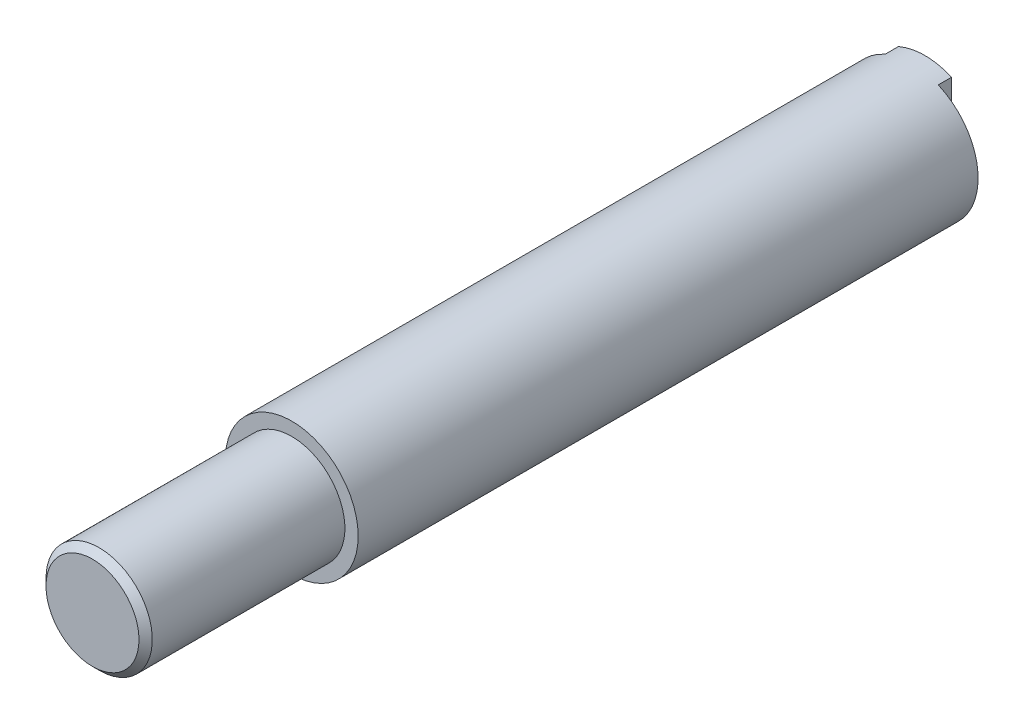
SolidWorks part; units mm, degrees
ref_plane "Front Plane" through (0, 0, 0) normal (0, 0, 1) x (1, 0, 0)
ref_plane "Top Plane" through (0, 0, 0) normal (0, 1, 0) x (1, 0, 0)
ref_plane "Right Plane" through (0, 0, 0) normal (1, 0, 0) x (0, 0, -1)
sketch "Sketch1" plane through (0, 0, 0) normal (0, 0, 1) x (1, 0, 0)
  circle A0 centre (0, 0) radius 15
  dimension "D1" = 30
extrude "Boss-Extrude1" add sketch "Sketch1" along normal blind 140
sketch "Sketch2" plane through (0, 0, 140) normal (0, 0, 1) x (1, 0, 0)
  circle A0 centre (0, 0) radius 12
  dimension "D1" = 24
extrude "Boss-Extrude2" add sketch "Sketch2" along normal blind 45
sketch "Sketch3" plane through (0, 0, 0) normal (0, 0, -1) x (-1, 0, 0)
  line L0 (0, 15) -> (0, -15) construction
  line L1 (-6, 13.7477) -> (-6, -13.7477)
  line L2 (6, 13.7477) -> (6, -13.7477)
  circle A0 centre (0, 0) radius 15 construction
  arc A1 (6, 13.7477) -> (-6, 13.7477) centre (0, 0) ccw
  arc A2 (-6, -13.7477) -> (6, -13.7477) centre (0, 0) ccw
  dimension "D2" = 30
  dimension "D1" = 12
extrude "Boss-Extrude3" add sketch "Sketch3" along normal blind 3
hole_wizard "M10 Tapped Hole1" positions "Sketch5" profile "Sketch4" tap size "M10" standard "GB"
sketch "Sketch5" plane through (0, 0, -3) normal (0, 0, -1) x (-1, 0, 0)
  point P0 (0, 0)
sketch "Sketch4" plane through (0, 0, -3) normal (1, 0, 0) x (0, 1, 0)
  line L0 (0, 0) -> (0, 27.0537)
  line L1 (0, 27.0537) -> (4.25, 24.5)
  line L2 (4.25, 24.5) -> (4.25, 0)
  line L5 (4.25, 0) -> (0, 0)
  line L10 (0, 27.0537) -> (-4.25, 24.5) construction
  line L11 (0, -6.35) -> (0, 107.95) construction
  dimension "螺纹孔钻头直径" = 8.5
  dimension "螺纹孔钻头深度" = 24.5
  dimension "导头角度" = 118
cosmetic thread "Cosmetic Thread1" parameters "D1"=20, "D2"=10
chamfer "Chamfer1" distance 1.5 angle 45 1 edges at (12, 0, 185)
